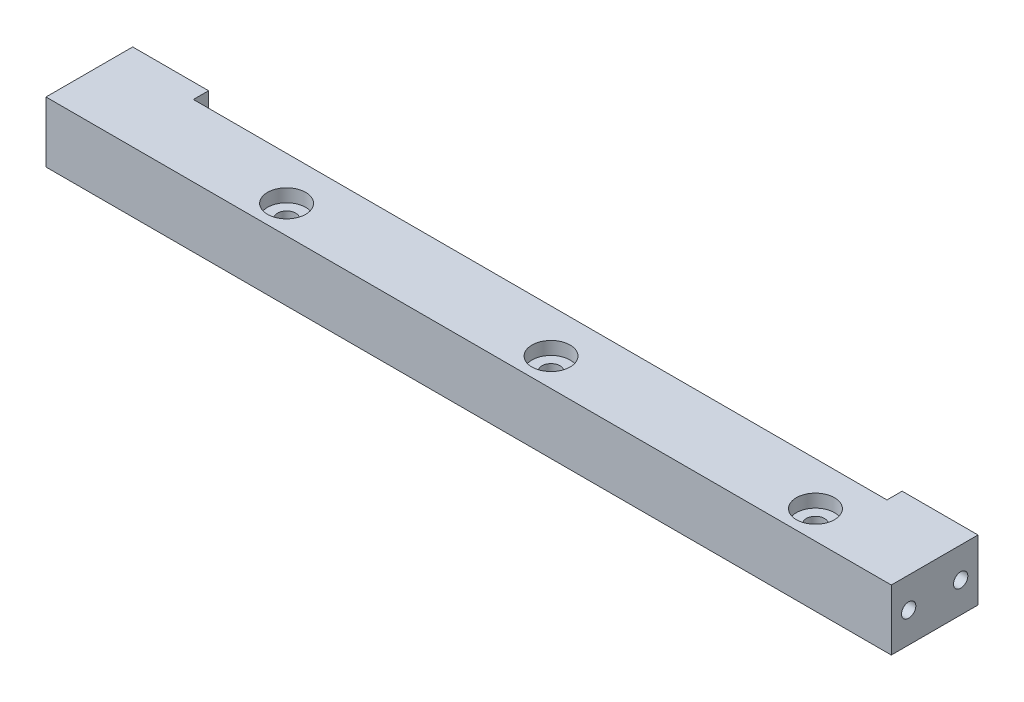
SolidWorks part; units mm, degrees
ref_plane "Front Plane" through (0, 0, 0) normal (0, 0, 1) x (1, 0, 0)
ref_plane "Top Plane" through (0, 0, 0) normal (0, 1, 0) x (1, 0, 0)
ref_plane "Right Plane" through (0, 0, 0) normal (1, 0, 0) x (0, 0, -1)
sketch "Sketch1" plane through (0, 0, 0) normal (0, 0, 1) x (1, 0, 0)
  line L1 (0, 0) -> (-195, 0)
  dimension "D2" = 195
extrude "Extrude-Thin1" add sketch "Sketch1" along normal mid plane 20 thin
hole_wizard "M4 Tapped Hole1" positions "Sketch2" profile "Sketch3" tap size "M4" standard "ISO"
sketch "Sketch2" plane through (-195, 0, 0) normal (-1, 0, 0) x (0, 0, 1)
  line L0 (0, 0) -> (0, -5.1315) construction
  line L1 (10, 0) -> (-10, 0) construction
  line L3 (-10, 7) -> (-6, 7) construction
  line L4 (-10, 0) -> (-10, 14) construction
  point P0 (-6, 7)
  point P2 (6, 7)
  dimension "D1" = 12
sketch "Sketch3" plane through (-195, 7, -6) normal (0, 1, 0) x (0, 0, 1)
  line L0 (0, 0) -> (0, 11.0914)
  line L1 (0, 11.0914) -> (1.65, 10.1)
  line L2 (1.65, 10.1) -> (1.65, 0)
  line L5 (1.65, 0) -> (0, 0)
  line L10 (0, 11.0914) -> (-1.65, 10.1) construction
  line L11 (0, -6.35) -> (0, 107.95) construction
  dimension "螺纹孔钻头直径" = 3.3
  dimension "螺纹孔钻头深度" = 10.1
  dimension "导头角度" = 118
cosmetic thread "Cosmetic Thread1" parameters "D1"=8, "D2"=4
cosmetic thread "Cosmetic Thread2" parameters "D1"=8, "D2"=4
hole_wizard "M4 Tapped Hole2" positions "Sketch4" profile "Sketch5" tap size "M4" standard "ISO"
sketch "Sketch4" plane through (0, 0, 0) normal (1, 0, 0) x (0, 0, -1)
  point P0 (-6, 7)
  point P3 (6, 7)
sketch "Sketch5" plane through (0, 7, 6) normal (0, 1, 0) x (0, 0, -1)
  line L0 (0, 0) -> (0, 11.0914)
  line L1 (0, 11.0914) -> (1.65, 10.1)
  line L2 (1.65, 10.1) -> (1.65, 0)
  line L5 (1.65, 0) -> (0, 0)
  line L10 (0, 11.0914) -> (-1.65, 10.1) construction
  line L11 (0, -6.35) -> (0, 107.95) construction
  dimension "螺纹孔钻头直径" = 3.3
  dimension "螺纹孔钻头深度" = 10.1
  dimension "导头角度" = 118
cosmetic thread "Cosmetic Thread3" parameters "D1"=8, "D2"=4
cosmetic thread "Cosmetic Thread4" parameters "D1"=8, "D2"=4
hole_wizard "M5 Tapped Hole1" positions "Sketch6" profile "Sketch8" tap size "M5" standard "ISO" end condition through all
sketch "Sketch6" plane through (0, 14, 0) normal (0, 1, 0) x (1, 0, 0)
  line L0 (0, -10) -> (-195, -10) construction
  line L1 (-195, -10) -> (-195, 10) construction
  point P0 (-146, -3.5)
  point P2 (-85, -3.5)
  point P4 (-24, -3.5)
  dimension "D1" = 6.5
  dimension "D2" = 49
  dimension "D3" = 61
  dimension "D4" = 61
sketch "Sketch8" plane through (-146, 14, 3.5) normal (1, 0, 0) x (0, 0, 1)
  line L0 (0, 0) -> (0, 14)
  line L1 (0, 14) -> (2.1, 14)
  line L2 (2.1, 14) -> (2.1, 0)
  line L5 (2.1, 0) -> (0, 0)
  line L11 (0, -6.35) -> (0, 107.95) construction
  dimension "通孔螺纹孔钻头直径" = 4.2
  dimension "通孔螺纹孔钻头深度" = 14
cosmetic thread "Cosmetic Thread5" parameters "D2"=5
cosmetic thread "Cosmetic Thread6" parameters "D2"=5
cosmetic thread "Cosmetic Thread7" parameters "D2"=5
sketch "Sketch9" plane through (0, 14, 0) normal (0, 1, 0) x (1, 0, 0)
  circle A0 centre (-146, -3.5) radius 4.4
  circle A1 centre (-85, -3.5) radius 4.4
  circle A2 centre (-24, -3.5) radius 4.4
  dimension "D1" = 8.8
extrude "Cut-Extrude1" cut sketch "Sketch9" against normal blind 3
sketch "Sketch10" plane through (0, 14, 0) normal (0, 1, 0) x (1, 0, 0)
  line L0 (0, 10) -> (-195, 10) construction
  line L1 (-177.5, 10) -> (-17.5, 10)
  line L2 (-177.5, 10) -> (-177.5, 6.5)
  line L3 (-177.5, 6.5) -> (-17.5, 6.5)
  line L4 (-17.5, 10) -> (-17.5, 6.5)
  line L5 (-97.5, -10) -> (-97.5, 6.5) construction
  line L6 (0, -10) -> (-195, -10) construction
  dimension "D1" = 160
  dimension "D2" = 3.5
extrude "Cut-Extrude2" cut sketch "Sketch10" against normal through all
